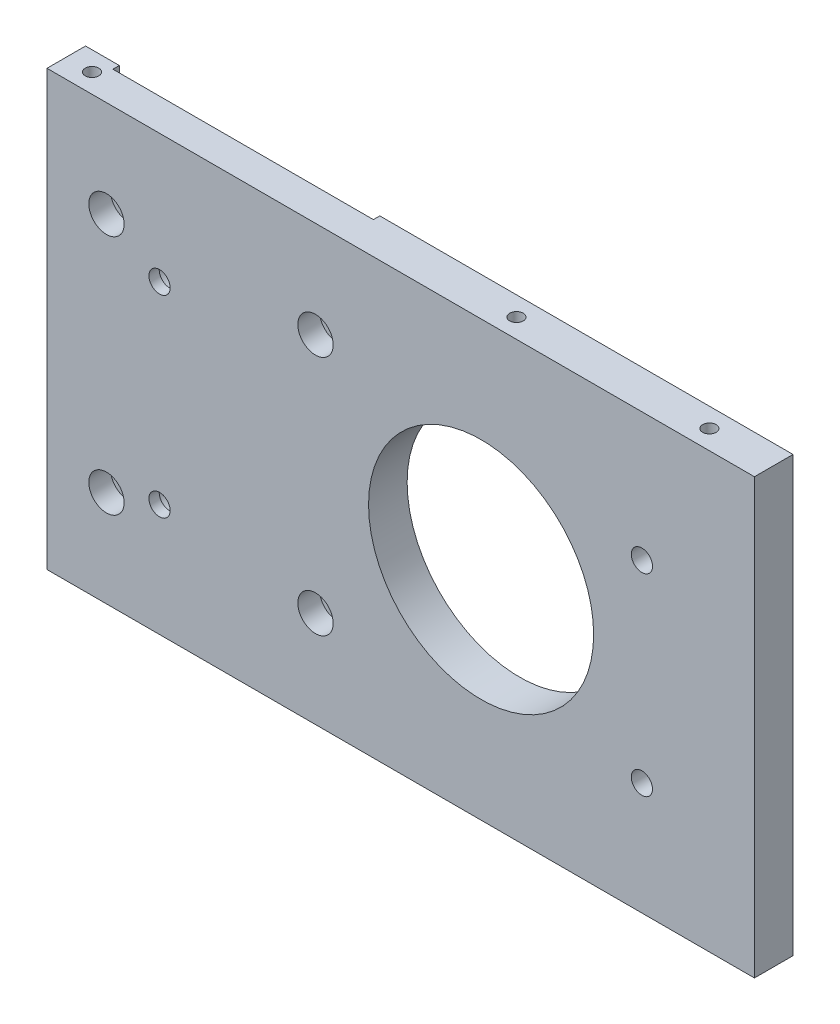
SolidWorks part; units mm, degrees
ref_plane "前视基准面" through (0, 0, 0) normal (0, 0, 1) x (1, 0, 0)
ref_plane "上视基准面" through (0, 0, 0) normal (0, 1, 0) x (1, 0, 0)
ref_plane "右视基准面" through (0, 0, 0) normal (1, 0, 0) x (0, 0, -1)
sketch "草图1" plane through (0, 0, 0) normal (0, 0, 1) x (1, 0, 0)
  line L1 (110, -67.5) -> (-110, -67.5)
  line L2 (110, -67.5) -> (110, 67.5)
  line L3 (110, 67.5) -> (-110, 67.5)
  line L4 (-110, -67.5) -> (-110, 67.5)
  line L5 (110, -67.5) -> (-110, 67.5) construction
  line L6 (110, 67.5) -> (-110, -67.5) construction
  point P0 (0, 0)
  dimension "D1" = 220
  dimension "D2" = 135
extrude "凸台-拉伸1" add sketch "草图1" along normal blind 12
hole_wizard "打孔尺寸(%根据)内六角圆柱头螺钉的类型1" positions "草图2" profile "草图3" counterbore size "M6" standard "GB" end condition up to next
sketch "草图2" plane through (0, 0, 12) normal (0, 0, 1) x (1, 0, 0)
  point P0 (-91.5, 37.5)
  point P3 (-26.5, 37.5)
  point P6 (-91.5, -37.5)
  point P9 (-26.5, -37.5)
sketch "草图3" plane through (-91.5, 37.5, 12) normal (1, 0, 0) x (0, -1, 0)
  line L0 (0, 0) -> (0, 12)
  line L1 (0, 12) -> (3.3, 12)
  line L3 (3.3, 12) -> (3.3, 6.8)
  line L4 (3.3, 6.8) -> (5.5, 6.8)
  line L5 (5.5, 6.8) -> (5.5, 0)
  line L7 (5.5, 0) -> (0, 0)
  line L11 (0, -6.35) -> (0, 107.95) construction
  dimension "通孔孔直径" = 6.6
  dimension "通孔孔深度" = 12
  dimension "柱形沉头孔直径" = 11
  dimension "柱形沉头孔深度" = 6.8
sketch "草图4" plane through (0, 0, 0) normal (0, 0, -1) x (-1, 0, 0)
  line L0 (26.5, 37.5) -> (91.5, 37.5) construction
  line L1 (26.5, -37.5) -> (91.5, -37.5) construction
  line L2 (59, -37.5) -> (59, 37.5) construction
  line L3 (-110, 67.5) -> (110, 67.5) construction
  line L4 (99.5, -67.5) -> (18.5, -67.5)
  line L5 (99.5, -67.5) -> (99.5, 67.5)
  line L6 (99.5, 67.5) -> (18.5, 67.5)
  line L7 (18.5, -67.5) -> (18.5, 67.5)
  line L8 (99.5, -67.5) -> (18.5, 67.5) construction
  line L9 (99.5, 67.5) -> (18.5, -67.5) construction
  point P10 (59, 0)
  dimension "D1" = 81
extrude "切除-拉伸1" cut sketch "草图4" against normal blind 2
hole_wizard "打孔尺寸(%根据)内六角圆柱头螺钉的类型2" positions "草图5" profile "草图6" counterbore size "M6" standard "GB" end condition up to next
sketch "草图5" plane through (0, 0, 2) normal (0, 0, -1) x (-1, 0, 0)
  point P0 (75, -32.5)
  point P3 (75, 27.5)
sketch "草图6" plane through (-75, -32.5, 2) normal (1, 0, 0) x (0, 1, 0)
  line L0 (0, 0) -> (0, 10)
  line L1 (0, 10) -> (3.3, 10)
  line L3 (3.3, 10) -> (3.3, 6.8)
  line L4 (3.3, 6.8) -> (5.5, 6.8)
  line L5 (5.5, 6.8) -> (5.5, 0)
  line L7 (5.5, 0) -> (0, 0)
  line L11 (0, -6.35) -> (0, 107.95) construction
  dimension "通孔孔直径" = 6.6
  dimension "通孔孔深度" = 10
  dimension "柱形沉头孔直径" = 11
  dimension "柱形沉头孔深度" = 6.8
hole_wizard "打孔尺寸(%根据)内六角圆柱头螺钉的类型3" positions "草图7" profile "草图8" counterbore size "M6" standard "GB" end condition up to next
sketch "草图7" plane through (0, 0, 0) normal (0, 0, -1) x (-1, 0, 0)
  point P0 (-75, -32.5)
  point P3 (-75, 27.5)
sketch "草图8" plane through (75, -32.5, 0) normal (1, 0, 0) x (0, 1, 0)
  line L0 (0, 0) -> (0, 12)
  line L1 (0, 12) -> (3.3, 12)
  line L3 (3.3, 12) -> (3.3, 6.8)
  line L4 (3.3, 6.8) -> (5.5, 6.8)
  line L5 (5.5, 6.8) -> (5.5, 0)
  line L7 (5.5, 0) -> (0, 0)
  line L11 (0, -6.35) -> (0, 107.95) construction
  dimension "通孔孔直径" = 6.6
  dimension "通孔孔深度" = 12
  dimension "柱形沉头孔直径" = 11
  dimension "柱形沉头孔深度" = 6.8
sketch "草图9" plane through (0, 0, 0) normal (0, 0, -1) x (-1, 0, 0)
  line L0 (-110, 0) -> (-25, 0) construction
  line L1 (-110, -67.5) -> (-110, 67.5) construction
  circle A0 centre (-25, 0) radius 35
  dimension "D1" = 70
  dimension "D2" = 85
extrude "切除-拉伸2" cut sketch "草图9" against normal up to next and the other way through all
hole_wizard "M5 螺纹孔1" positions "草图10" profile "草图12" tap size "M5" standard "GB"
sketch "草图10" plane through (0, 67.5, 0) normal (0, 1, 0) x (1, 0, 0)
  line L0 (110, -6) -> (90, -6) construction
  line L1 (110, -12) -> (110, 0) construction
  line L2 (90, -6) -> (30, -6) construction
  line L4 (-102, -6) -> (30, -6) construction
  point P0 (90, -6)
  point P2 (30, -6)
  point P16 (-102, -6)
  dimension "D1" = 20
  dimension "D2" = 60
  dimension "D3" = 132
sketch "草图12" plane through (90, 67.5, 6) normal (1, 0, 0) x (0, 0, 1)
  line L0 (0, 0) -> (0, 13.6618)
  line L1 (0, 13.6618) -> (2.1, 12.4)
  line L2 (2.1, 12.4) -> (2.1, 0)
  line L5 (2.1, 0) -> (0, 0)
  line L10 (0, 13.6618) -> (-2.1, 12.4) construction
  line L11 (0, -6.35) -> (0, 107.95) construction
  dimension "螺纹孔钻头直径" = 4.2
  dimension "螺纹孔钻头深度" = 12.4
  dimension "导头角度" = 118
cosmetic thread "孔螺蚊线1" parameters "D1"=10, "D2"=5
cosmetic thread "孔螺蚊线2" parameters "D1"=10, "D2"=5
cosmetic thread "孔螺蚊线3" parameters "D1"=10, "D2"=5
